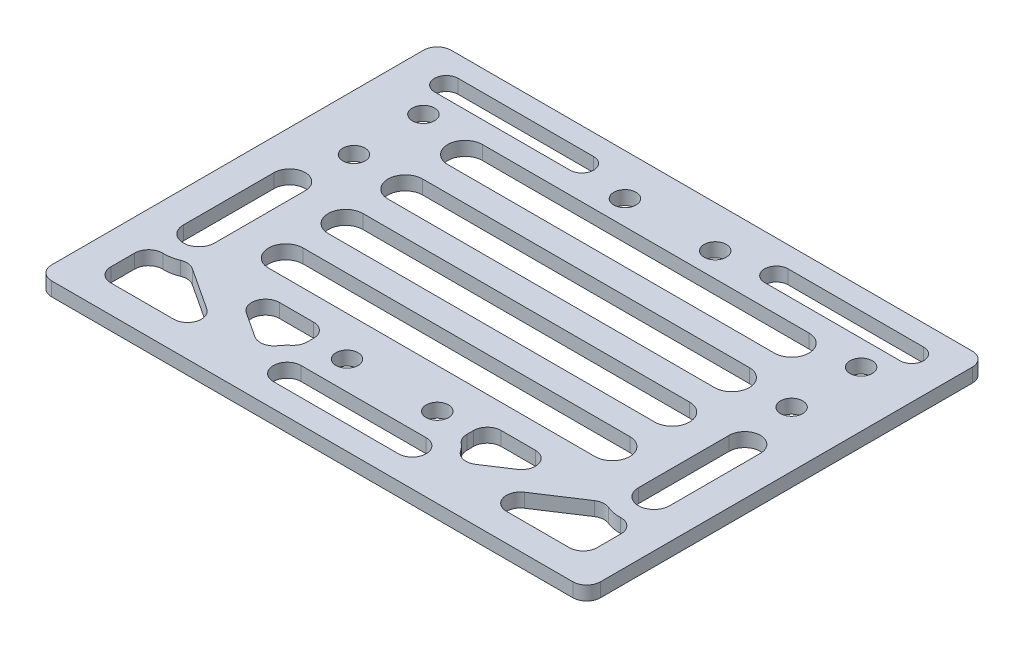
from build123d import *

# Parameters (mm, degrees)
SKETCH_1_W          = 79
SKETCH_1_H          = 57.5
SKETCH_1_R          = 1.6
EXTRUDE_1_DEPTH     = 2
CUT_EXTRUDE_1_DEPTH = 49.895935414
FILLET_R2_1_R       = 2


with BuildPart() as part:
    # 草图1 → 凸台-拉伸1 (new body)
    with BuildSketch(Plane(origin=(0, 0, 0), x_dir=(1, 0, 0), z_dir=(0, 1, 0))):
        Rectangle(SKETCH_1_W, SKETCH_1_H)
        with Locations(Location((-31.5, 18.75, 0), (0, 0, 270))):
            Circle(SKETCH_1_R, mode=Mode.SUBTRACT)
        with Locations(Location((-31.5, 8.75, 0), (0, 0, 270))):
            Circle(SKETCH_1_R, mode=Mode.SUBTRACT)
        with Locations(Location((31.5, 8.75, 0), (0, 0, 90))):
            Circle(SKETCH_1_R, mode=Mode.SUBTRACT)
        with Locations(Location((31.5, 18.75, 0), (0, 0, 90))):
            Circle(SKETCH_1_R, mode=Mode.SUBTRACT)
        with Locations(Location((-6.5, 22.75, 0), (0, 0, 270))):
            Circle(SKETCH_1_R, mode=Mode.SUBTRACT)
        with Locations(Location((-6.5, -17.25, 0), (0, 0, 270))):
            Circle(SKETCH_1_R, mode=Mode.SUBTRACT)
        with Locations(Location((6.5, 22.75, 0), (0, 0, 90))):
            Circle(SKETCH_1_R, mode=Mode.SUBTRACT)
        with Locations(Location((6.5, -17.25, 0), (0, 0, 90))):
            Circle(SKETCH_1_R, mode=Mode.SUBTRACT)
    extrude(amount=EXTRUDE_1_DEPTH)

    # 草图2 → 切除-拉伸1 (cut, through all)
    with BuildSketch(Plane(origin=(0, 2, 0), x_dir=(1, 0, 0), z_dir=(0, 1, 0))):
        with BuildLine():
            Line((-23.5, 19.25), (23.5, 19.25))
            ThreePointArc((23.5, 19.25), (26, 16.75), (23.5, 14.25))
            Line((23.5, 14.25), (-23.5, 14.25))
            ThreePointArc((-23.5, 14.25), (-26, 16.75), (-23.5, 19.25))
        make_face()
        with BuildLine():
            Line((-23.5, 10.65), (23.5, 10.65))
            ThreePointArc((23.5, 10.65), (26, 8.15), (23.5, 5.65))
            Line((23.5, 5.65), (-23.5, 5.65))
            ThreePointArc((-23.5, 5.65), (-26, 8.15), (-23.5, 10.65))
        make_face()
        with BuildLine():
            Line((-23.5, 2.05), (23.5, 2.05))
            ThreePointArc((23.5, 2.05), (26, -0.45), (23.5, -2.95))
            Line((23.5, -2.95), (-23.5, -2.95))
            ThreePointArc((-23.5, -2.95), (-26, -0.45), (-23.5, 2.05))
        make_face()
        with BuildLine():
            Line((-23.5, -6.55), (23.5, -6.55))
            ThreePointArc((23.5, -6.55), (26, -9.05), (23.5, -11.55))
            Line((23.5, -11.55), (-23.5, -11.55))
            ThreePointArc((-23.5, -11.55), (-26, -9.05), (-23.5, -6.55))
        make_face()
        with BuildLine():
            Line((-33.5, 25.75), (-14, 25.75))
            ThreePointArc((-14, 25.75), (-12.3, 24.05), (-14, 22.35))
            Line((-14, 22.35), (-33.5, 22.35))
            ThreePointArc((-33.5, 22.35), (-35.2, 24.05), (-33.5, 25.75))
        make_face()
        with BuildLine():
            Line((33.5, 25.75), (14, 25.75))
            ThreePointArc((14, 25.75), (12.3, 24.05), (14, 22.35))
            Line((14, 22.35), (33.5, 22.35))
            ThreePointArc((33.5, 22.35), (35.2, 24.05), (33.5, 25.75))
        make_face()
        with BuildLine():
            Line((-9, -21.35), (9, -21.35))
            ThreePointArc((9, -21.35), (11, -23.35), (9, -25.35))
            Line((9, -25.35), (-9, -25.35))
            ThreePointArc((-9, -25.35), (-11, -23.35), (-9, -21.35))
        make_face()
        with BuildLine():
            Line((-30.5, 0.75), (-30.5, -12.305379368))
            ThreePointArc((-30.5, -12.305379368), (-32.75, -14.555379368), (-35, -12.305379368))
            Line((-35, -12.305379368), (-35, 0.75))
            ThreePointArc((-35, 0.75), (-32.75, 3), (-30.5, 0.75))
        make_face()
        with BuildLine():
            Line((30.5, 0.75), (30.5, -12.305379368))
            ThreePointArc((30.5, -12.305379368), (32.75, -14.555379368), (35, -12.305379368))
            Line((35, -12.305379368), (35, 0.75))
            ThreePointArc((35, 0.75), (32.75, 3), (30.5, 0.75))
        make_face()
        with BuildLine():
            Line((-35, -16.770522143), (-35, -24.75))
            Line((-35, -24.75), (-17.261316253, -24.75))
            Line((-17.261316253, -24.75), (-29.927103479, -16.432273507))
            ThreePointArc((-29.927103479, -16.432273507), (-32.417350574, -17.294301533), (-35, -16.770522143))
        make_face()
        with BuildLine():
            Line((-25.10932284, -15.05), (-11.5, -15.05))
            Line((-11.5, -15.05), (-11.5, -19.019872981))
            ThreePointArc((-11.5, -19.019872981), (-13.073188505, -20.450149072), (-13.909844854, -22.404789172))
            Line((-13.909844854, -22.404789172), (-25.10932284, -15.05))
        make_face()
        with BuildLine():
            Line((17.261316253, -24.75), (29.927103479, -16.432273507))
            ThreePointArc((29.927103479, -16.432273507), (32.417350574, -17.294301533), (35, -16.770522143))
            Line((35, -16.770522143), (35, -24.75))
            Line((35, -24.75), (17.261316253, -24.75))
        make_face()
        with BuildLine():
            Line((25.10932284, -15.05), (11.5, -15.05))
            Line((11.5, -15.05), (11.5, -19.019872981))
            ThreePointArc((11.5, -19.019872981), (13.073188505, -20.450149072), (13.909844854, -22.404789172))
            Line((13.909844854, -22.404789172), (25.10932284, -15.05))
        make_face()
    extrude(amount=-CUT_EXTRUDE_1_DEPTH, mode=Mode.SUBTRACT)

    # R2 圆角1
    fillet_r2_1_edges = [part.edges().sort_by_distance(p)[0] for p in [
        (-11.5, 1, 15.05),
        (-11.5, 1, 19.019872981),
        (-13.909844854, 1, 22.404789172),
        (-25.10932284, 1, 15.05),
        (-35, 1, 16.770522143),
        (-29.927103479, 1, 16.432273507),
        (-17.261316253, 1, 24.75),
        (-35, 1, 24.75),
        (25.10932284, 1, 15.05),
        (13.909844854, 1, 22.404789172),
        (11.5, 1, 19.019872981),
        (11.5, 1, 15.05),
        (29.927103479, 1, 16.432273507),
        (35, 1, 16.770522143),
        (35, 1, 24.75),
        (17.261316253, 1, 24.75),
        (39.5, 1, 28.75),
        (-39.5, 1, 28.75),
        (-39.5, 1, -28.75),
        (39.5, 1, -28.75),
    ]]
    fillet(fillet_r2_1_edges, radius=FILLET_R2_1_R)


solid = part.part
